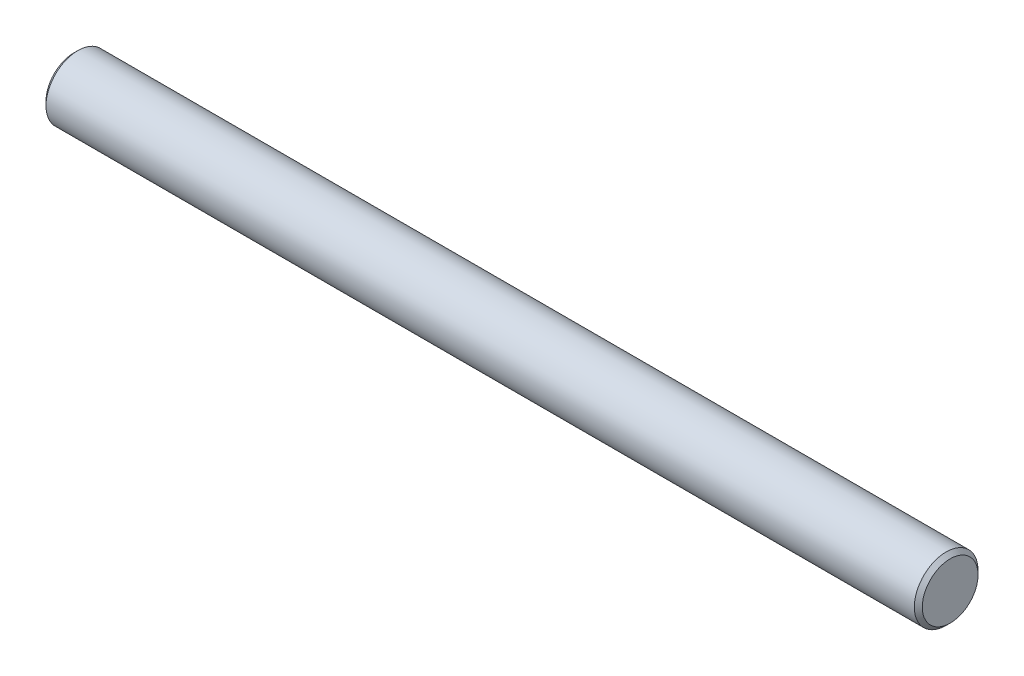
from build123d import *

# Parameters (mm, degrees)
SKETCH1_W          = 110
SKETCH1_H          = 4
SKETCH2_W          = 4
SKETCH2_H          = 2
CUT_EXTRUDE1_DEPTH = 5
CHAMFER1_SIZE      = 0.5


with BuildPart() as part:
    # Sketch1 → Revolve1 (revolve)
    with BuildSketch(Plane.XY, mode=Mode.PRIVATE) as revolve1_sk:
        with Locations((55, 2)):
            Rectangle(SKETCH1_W, SKETCH1_H)
    revolve(revolve1_sk.sketch.rotate(Axis((0, 0, 0), (1, 0, 0)), 90), axis=Axis((0, 0, 0), (1, 0, 0)))

    # Sketch2 → Cut-Extrude1 (cut, symmetric)
    with BuildSketch(Plane(origin=(0, 0, 0), x_dir=(1, 0, 0), z_dir=(0, 1, 0))):
        with Locations((4, 4)):
            Rectangle(SKETCH2_W, SKETCH2_H)
    extrude(amount=CUT_EXTRUDE1_DEPTH, both=True, mode=Mode.SUBTRACT)

    # Chamfer1
    chamfer1_edges = [part.edges().sort_by_distance(p)[0] for p in [
        (110, 0, -4),
        (0, 0, -4),
    ]]
    chamfer(chamfer1_edges, length=CHAMFER1_SIZE)


solid = part.part
